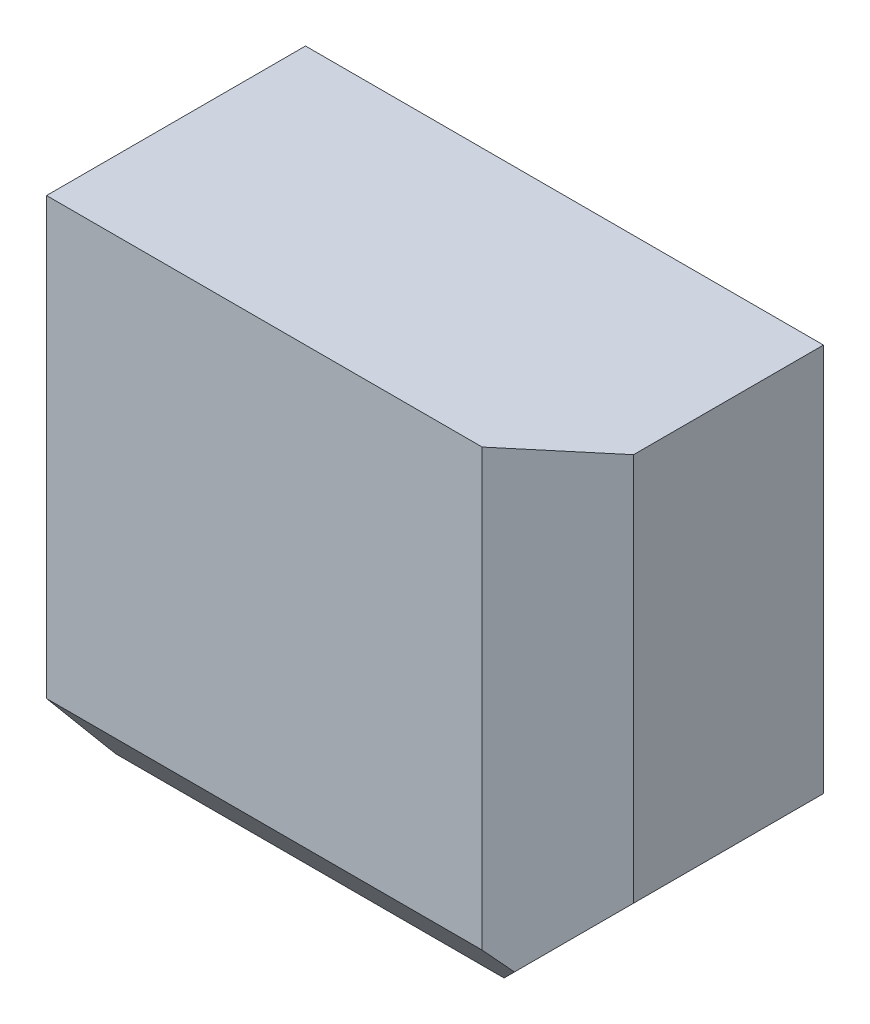
from build123d import *

# Parameters (mm, degrees)
SKETCH1_W           = 60
SKETCH1_H           = 60
BOSS_EXTRUDE1_DEPTH = 15
CHAMFER1_SIZE       = 15
CHAMFER2_SIZE       = 8
CHAMFER2_SIZE2      = 9.534028741
CHAMFER3_SIZE       = 8
CHAMFER3_SIZE2      = 9.534028741


with BuildPart() as part:
    # Sketch1 → Boss-Extrude1 (new, symmetric)
    with BuildSketch(Plane.XY):
        Rectangle(SKETCH1_W, SKETCH1_H)
    extrude(amount=BOSS_EXTRUDE1_DEPTH, both=True)

    # Chamfer1
    chamfer1_edges = [part.edges().sort_by_distance(p)[0] for p in [
        (30, -30, 0),
    ]]
    chamfer(chamfer1_edges, length=CHAMFER1_SIZE)

    # Chamfer2
    chamfer2_edges = [part.edges().sort_by_distance(p)[0] for p in [
        (-7.5, -30, 15),
    ]]
    chamfer2_side = [part.faces().sort_by_distance(p)[0] for p in [
        (-7.5, -30, 0),
    ]]
    chamfer(chamfer2_edges, length=CHAMFER2_SIZE, length2=CHAMFER2_SIZE2, reference=chamfer2_side[0])

    # Chamfer3
    chamfer3_edges = [part.edges().sort_by_distance(p)[0] for p in [
        (30, 7.5, 15),
    ]]
    chamfer3_side = [part.faces().sort_by_distance(p)[0] for p in [
        (30, 7.5, 0),
    ]]
    chamfer(chamfer3_edges, length=CHAMFER3_SIZE, length2=CHAMFER3_SIZE2, reference=chamfer3_side[0])


solid = part.part
